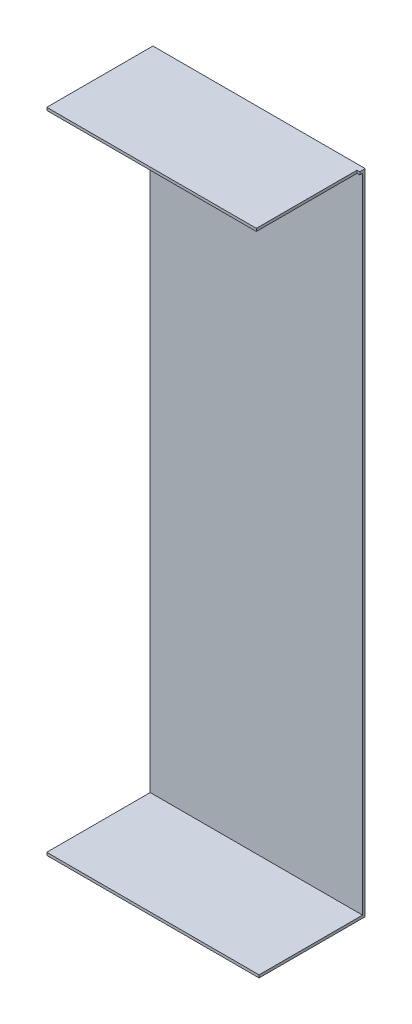
SolidWorks part; units mm, degrees
ref_plane "Front Plane" through (0, 0, 0) normal (0, 0, 1) x (1, 0, 0)
ref_plane "Top Plane" through (0, 0, 0) normal (0, 1, 0) x (1, 0, 0)
ref_plane "Right Plane" through (0, 0, 0) normal (1, 0, 0) x (0, 0, -1)
sketch "Sketch1" plane through (0, 0, 0) normal (0, 0, 1) x (1, 0, 0)
  line L1 (-38.5, 119) -> (38.5, 119)
  line L2 (-38.5, 119) -> (-38.5, -119)
  line L3 (-38.5, -119) -> (38.5, -119)
  line L4 (38.5, 119) -> (38.5, -119)
  line L5 (-38.5, 119) -> (38.5, -119) construction
  line L6 (-38.5, -119) -> (38.5, 119) construction
  point P0 (0, 0)
  dimension "D1" = 77
  dimension "D2" = 238
extrude "Boss-Extrude1" add sketch "Sketch1" along normal blind 1
sketch "Sketch2" plane through (0, 0, 1) normal (0, 0, 1) x (1, 0, 0)
  line L0 (38.5, -119) -> (38.5, 119) construction
  line L1 (-38.5, 119) -> (38.5, 119)
  line L2 (-38.5, 119) -> (-38.5, 118)
  line L3 (-38.5, 118) -> (38.5, 118)
  line L4 (38.5, 119) -> (38.5, 118)
  line L5 (0, 0) -> (88.4377, 0) construction
  line L6 (38.5, -119) -> (38.5, -118)
  line L7 (-38.5, -118) -> (38.5, -118)
  line L8 (-38.5, -119) -> (-38.5, -118)
  line L9 (-38.5, -119) -> (38.5, -119)
  dimension "D1" = 1
extrude "Boss-Extrude2" add sketch "Sketch2" along normal blind 38
sketch "Sketch3" plane through (38.5, 0, 0) normal (1, 0, 0) x (0, 0, -1)
  line L0 (-2, 119) -> (-2, 118)
  line L8 (0, -119) -> (0, 119)
  line L9 (0, 119) -> (-39, 119)
  line L10 (-39, 119) -> (-39, 118)
  line L11 (-39, 118) -> (-1, 118)
  line L12 (-1, 118) -> (-1, -118)
  line L13 (-1, -118) -> (-39, -118)
  line L14 (-39, -118) -> (-39, -119)
  line L15 (-39, -119) -> (0, -119)
  line L16 (0, -119) -> (0, 119)
  line L17 (0, 119) -> (-2, 119)
  line L19 (-2, 118) -> (-1, 118)
  line L20 (-1, 118) -> (-1, -118)
  line L21 (-1, -118) -> (-39, -118)
  line L22 (-39, -118) -> (-39, -119)
  line L23 (-39, -119) -> (0, -119)
  dimension "D1" = 0
extrude "Boss-Extrude3" add sketch "Sketch3" along normal blind 1
